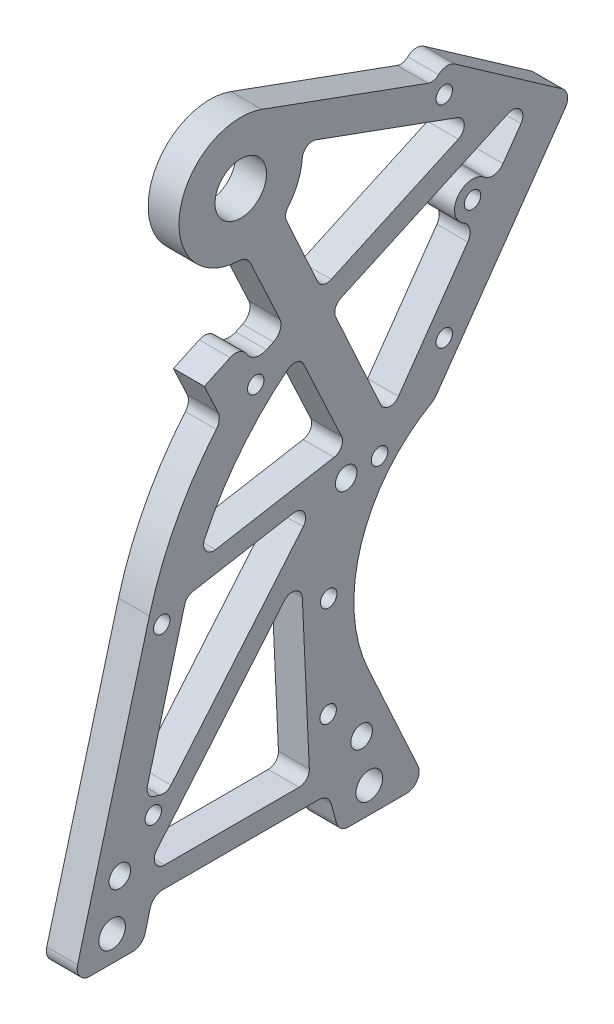
from build123d import *

# Parameters (mm, degrees)
SKETCH_1_R          = 5
SKETCH_1_R_2        = 2.6
EXTRUDE_1_DEPTH     = 6
SKETCH_2_R          = 1.6
SKETCH_2_R_2        = 2.1
CUT_EXTRUDE_1_DEPTH = 139.597884305
CUT_EXTRUDE_2_DEPTH = 139.597884305
FILLET_R2_5_1_R     = 2.5


with BuildPart() as part:
    # 草图1 → 凸台-拉伸1 (new body)
    with BuildSketch(Plane(origin=(0, 0, 0), x_dir=(0, 0, -1), z_dir=(1, 0, 0))):
        with BuildLine():
            Line((-17.083193756, 0), (17.083193756, 0))
            Line((17.083193756, 0), (19.092812699, -7.5))
            Line((19.092812699, -7.5), (36.089714585, -7.5))
            Line((36.089714585, -7.5), (24.725322655, 17.309358564))
            ThreePointArc((24.725322655, 17.309358564), (23.529105799, 39.258626053), (37.618636127, 56.131278873))
            Line((37.618636127, 56.131278873), (64.553261218, 94.597910009))
            Line((64.553261218, 94.597910009), (41.617003978, 110.658050227))
            ThreePointArc((41.617003978, 110.658050227), (40.005403895, 111.103849583), (38.473281109, 110.434079727))
            ThreePointArc((38.473281109, 110.434079727), (37.50675935, 109.933882183), (36.421415399, 110.013822175))
            Line((36.421415399, 110.013822175), (4.10424172, 121.776311449))
            ThreePointArc((4.10424172, 121.776311449), (-11.904439355, 112.011397909), (1.156148672, 98.55582484))
            Line((1.156148672, 98.55582484), (8.630698442, 82.526601129))
            Line((8.630698442, 82.526601129), (5.005467294, 80.836128082))
            ThreePointArc((5.005467294, 80.836128082), (2.840887568, 80.692205939), (1.145207204, 82.045271746))
            ThreePointArc((1.145207204, 82.045271746), (-0.267859766, 83.172826585), (-2.071676205, 83.052891466))
            Line((-2.071676205, 83.052891466), (-7.077009672, 80.718866138))
            Line((-7.077009672, 80.718866138), (-3.722354698, 73.52478533))
            ThreePointArc((-3.722354698, 73.52478533), (-12.249590693, 61.281233983), (-17.760304381, 47.415797172))
            Line((-17.760304381, 47.415797172), (-32.561769984, -7.5))
            Line((-32.561769984, -7.5), (-19.092812699, -7.5))
            Line((-19.092812699, -7.5), (-17.083193756, 0))
        make_face()
        with Locations((0, 110.5)):
            Circle(SKETCH_1_R, mode=Mode.SUBTRACT)
        with Locations((-25, -2.5)):
            Circle(SKETCH_1_R_2, mode=Mode.SUBTRACT)
        with Locations((25, -2.5)):
            Circle(SKETCH_1_R_2, mode=Mode.SUBTRACT)
    extrude(amount=EXTRUDE_1_DEPTH)

    # 草图2 → 切除-拉伸1 (cut, through all)
    with BuildSketch(Plane(origin=(6, 0, 0), x_dir=(0, 0, -1), z_dir=(1, 0, 0))):
        with Locations((-17, 13.5)):
            Circle(SKETCH_2_R)
        with Locations((17, 13.5)):
            Circle(SKETCH_2_R)
        with Locations((39.580501258, 106.551942354)):
            Circle(SKETCH_2_R)
        with Locations((45.073459702, 86.051942354)):
            Circle(SKETCH_2_R)
        with Locations((39.580501258, 65.551942354)):
            Circle(SKETCH_2_R)
        with Locations((27.001946929, 51.949244407)):
            Circle(SKETCH_2_R)
        with Locations((17.106548453, 32.940360797)):
            Circle(SKETCH_2_R)
        with Locations((2.918948689, 76.032242648)):
            Circle(SKETCH_2_R)
        with Locations((-15.340180452, 44.750004318)):
            Circle(SKETCH_2_R)
        with Locations((-23.5, 6.5)):
            Circle(SKETCH_2_R_2)
        with Locations((23.5, 6.5)):
            Circle(SKETCH_2_R_2)
        with Locations((20.5, 51.5)):
            Circle(SKETCH_2_R_2)
    extrude(amount=-CUT_EXTRUDE_1_DEPTH, mode=Mode.SUBTRACT)

    # 草图3 → 切除-拉伸2 (cut, through all)
    with BuildSketch(Plane(origin=(6, 0, 0), x_dir=(0, 0, -1), z_dir=(1, 0, 0))):
        with BuildLine():
            Line((12.248429119, 74.768352656), (19.611098021, 58.979058243))
            ThreePointArc((19.611098021, 58.979058243), (19.571846918, 57.209063128), (18.142977061, 56.163714245))
            Line((18.142977061, 56.163714245), (-4.884471281, 52.137115682))
            ThreePointArc((-4.884471281, 52.137115682), (-6.818374298, 52.893229365), (-7.039018719, 54.957933901))
            ThreePointArc((-7.039018719, 54.957933901), (-0.107884381, 66.158502025), (9.190257276, 75.487913111))
            ThreePointArc((9.190257276, 75.487913111), (10.893886548, 75.869951802), (12.248429119, 74.768352656))
        make_face()
        with BuildLine():
            Line((8.888031445, 100.650995125), (14.939630847, 87.381560906))
            ThreePointArc((14.939630847, 87.381560906), (16.059423219, 86.337908285), (17.589209845, 86.391747219))
            Line((17.589209845, 86.391747219), (42.297774007, 97.660225561))
            ThreePointArc((42.297774007, 97.660225561), (43.466338702, 99.558713974), (42.151931639, 101.359307145))
            Line((42.151931639, 101.359307145), (14.64760953, 111.370061707))
            ThreePointArc((14.64760953, 111.370061707), (12.876257738, 111.169293065), (11.968773637, 109.634865542))
            ThreePointArc((11.968773637, 109.634865542), (11.116698186, 105.981258866), (9.17805239, 102.769323811))
            ThreePointArc((9.17805239, 102.769323811), (8.726212744, 101.752167532), (8.888031445, 100.650995125))
        make_face()
        with BuildLine():
            Line((19.456445818, 82.297430448), (52.030599002, 97.153054484))
            ThreePointArc((52.030599002, 97.153054484), (54.397990964, 96.612445758), (54.498785746, 94.186205269))
            Line((54.498785746, 94.186205269), (48.555557448, 85.698395622))
            ThreePointArc((48.555557448, 85.698395622), (42.206427547, 88.059459881), (46.596632527, 82.900760901))
            Line((46.596632527, 82.900760901), (30.669808994, 60.154899618))
            ThreePointArc((30.669808994, 60.154899618), (28.848773175, 59.310417706), (27.211808562, 60.472169836))
            Line((27.211808562, 60.472169836), (18.466632131, 79.647851451))
            ThreePointArc((18.466632131, 79.647851451), (18.412793197, 81.177638076), (19.456445818, 82.297430448))
        make_face()
        with BuildLine():
            Line((10.282764815, 50.728578892), (-9.313741825, 47.301917619))
            ThreePointArc((-9.313741825, 47.301917619), (-10.318290453, 46.808320331), (-10.9003335, 45.852296211))
            Line((-10.9003335, 45.852296211), (-18.148908609, 18.958926922))
            ThreePointArc((-18.148908609, 18.958926922), (-17.895966668, 17.350400621), (-16.530693392, 16.463064513))
            ThreePointArc((-16.530693392, 16.463064513), (-16.184608866, 16.387063785), (-15.849899102, 16.270788322))
            ThreePointArc((-15.849899102, 16.270788322), (-14.608512176, 16.17512065), (-13.551076283, 16.832405317))
            Line((-13.551076283, 16.832405317), (12.159348315, 47.472896199))
            ThreePointArc((12.159348315, 47.472896199), (12.36002095, 49.757239414), (10.282764815, 50.728578892))
        make_face()
        with BuildLine():
            Line((-14.808099853, 4), (11.338749368, 4))
            ThreePointArc((11.338749368, 4), (12.78509952, 4.618670482), (13.336635527, 6.091928763))
            Line((13.336635527, 6.091928763), (11.977378786, 35.632631153))
            ThreePointArc((11.977378786, 35.632631153), (10.620148339, 37.435315876), (8.447403741, 36.82627761))
            Line((8.447403741, 36.82627761), (-16.340188739, 7.285575219))
            ThreePointArc((-16.340188739, 7.285575219), (-16.620715427, 5.154763477), (-14.808099853, 4))
        make_face()
    extrude(amount=-CUT_EXTRUDE_2_DEPTH, mode=Mode.SUBTRACT)

    # R2.5 圆角1
    fillet_r2_5_1_edges = [part.edges().sort_by_distance(p)[0] for p in [
        (3, 85.698395622, -48.555557448),
        (3, 82.900760901, -46.596632527),
        (3, -7.5, 19.092812699),
        (3, -7.5, 32.561769984),
        (3, 73.52478533, 3.722354698),
        (3, 82.526601129, -8.630698442),
        (3, 98.55582484, -1.156148672),
        (3, 94.597910009, -64.553261218),
        (3, 56.131278873, -37.618636127),
        (3, -7.5, -36.089714585),
        (3, -7.5, -19.092812699),
        (3, 0, -17.083193756),
        (3, 0, 17.083193756),
    ]]
    fillet(fillet_r2_5_1_edges, radius=FILLET_R2_5_1_R)


solid = part.part
